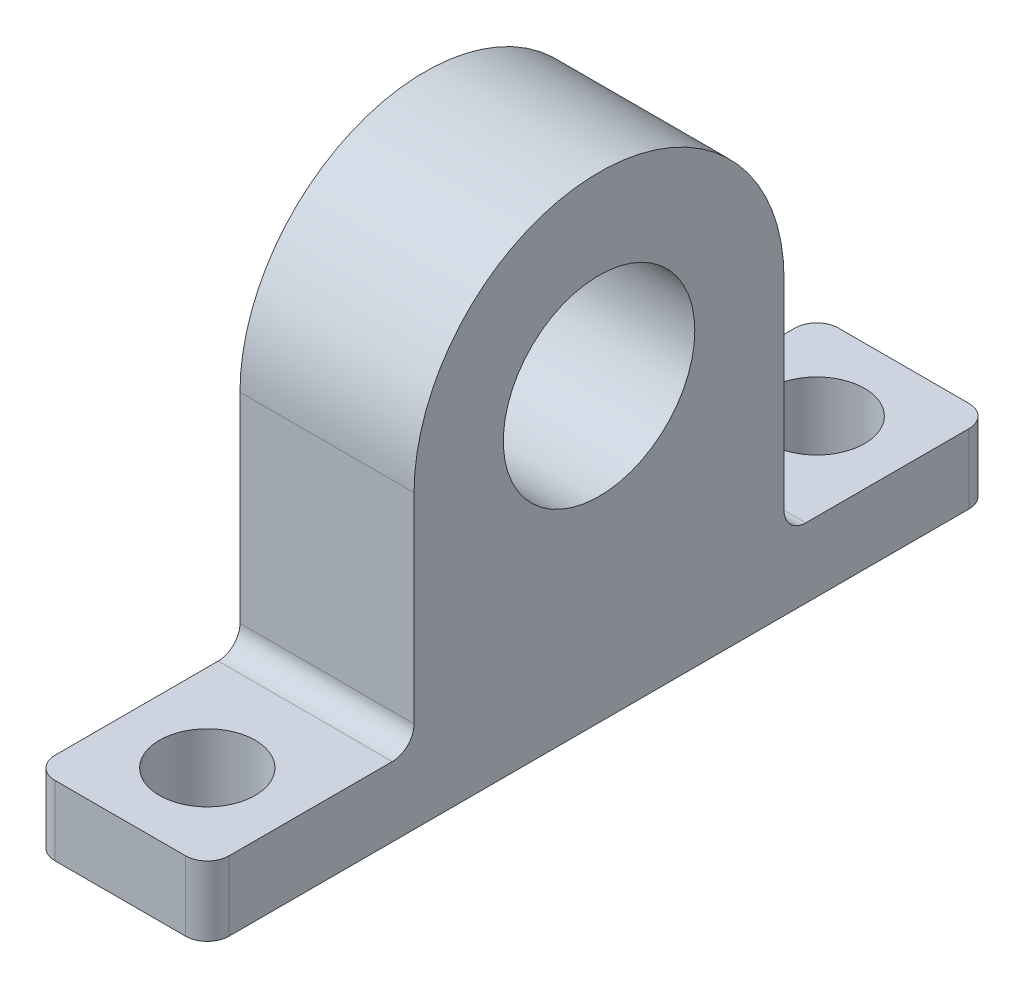
SolidWorks part; units mm, degrees
material "普通碳钢"
ref_plane "Front Plane" through (0, 0, 0) normal (0, 0, 1) x (1, 0, 0)
ref_plane "Top Plane" through (0, 0, 0) normal (0, 1, 0) x (1, 0, 0)
ref_plane "Right Plane" through (0, 0, 0) normal (1, 0, 0) x (0, 0, -1)
sketch "Sketch1" plane through (0, 0, 0) normal (0, 1, 0) x (1, 0, 0)
  line L0 (0, 90) -> (0, 0) construction
  line L1 (-20, 90) -> (20, 90)
  line L2 (-20, 90) -> (-20, -90)
  line L3 (-20, -90) -> (20, -90)
  line L4 (20, 90) -> (20, -90)
  line L5 (0, 0) -> (-20, 0) construction
  circle A0 centre (0, 70) radius 11
  circle A1 centre (0, -70) radius 11
  dimension "D3" = 22
  dimension "D1" = 180
  dimension "D2" = 40
  dimension "D4" = 140
extrude "Boss-Extrude1" add sketch "Sketch1" along normal blind 16
sketch "Sketch2" plane through (0, 0, 0) normal (1, 0, 0) x (0, 0, -1)
  line L0 (0, 8.8) -> (0, -8.8) construction
  line L1 (-42.5, 67) -> (-42.5, 16)
  line L2 (-90, 16) -> (90, 16) construction
  line L3 (42.5, 67) -> (42.5, 16)
  line L4 (-42.5, 16) -> (42.5, 16)
  line L5 (22, 0) -> (-22, 0) construction
  circle A0 centre (0, 67) radius 22
  arc A1 (42.5, 67) -> (-42.5, 67) centre (0, 67) ccw
  dimension "D2" = 44
  dimension "D3" = 67
  dimension "D1" = 85
extrude "Boss-Extrude2" add sketch "Sketch2" along normal mid plane 40
fillet "Fillet1" radius 5 6 edges at (20, 8, 90) (-20, 8, 90) (20, 8, -90) (-20, 8, -90)
